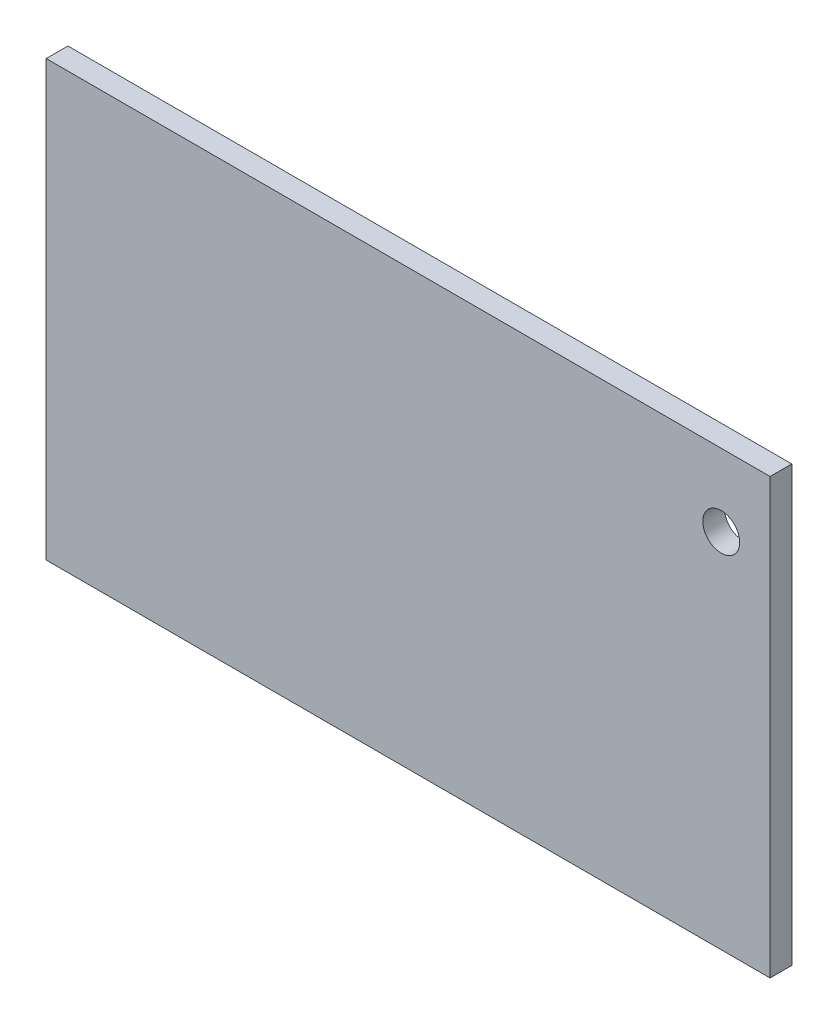
SolidWorks part; units mm, degrees
material "1023 碳钢板 (SS)"
ref_plane "Front Plane" through (0, 0, 0) normal (0, 0, 1) x (1, 0, 0)
ref_plane "Top Plane" through (0, 0, 0) normal (0, 1, 0) x (1, 0, 0)
ref_plane "Right Plane" through (0, 0, 0) normal (1, 0, 0) x (0, 0, -1)
sketch "Sketch1" plane through (0, 0, 0) normal (0, 0, 1) x (1, 0, 0)
  line L1 (100, 60) -> (-100, 60)
  line L2 (100, 60) -> (100, -60)
  line L3 (100, -60) -> (-100, -60)
  line L4 (-100, 60) -> (-100, -60)
  line L5 (100, 60) -> (-100, -60) construction
  line L6 (100, -60) -> (-100, 60) construction
  point P0 (0, 0)
  dimension "D1" = 200
  dimension "D2" = 120
extrude "Boss-Extrude1" add sketch "Sketch1" along normal blind 6
sketch "Sketch2" plane through (0, 0, 6) normal (0, 0, 1) x (1, 0, 0)
  line L0 (100, 60) -> (-100, 60) construction
  line L1 (100, -60) -> (100, 60) construction
  circle A0 centre (86.5, 40) radius 4.5
  dimension "D1" = 20
  dimension "D2" = 13.5
  dimension "D3" = 9
hole_wizard "M12 Tapped Hole1" positions "Sketch3" profile "Sketch4" tap size "M12" standard "ISO"
sketch "Sketch3" plane through (0, 0, 6) normal (0, 0, 1) x (1, 0, 0)
  point P0 (86.5, 40)
sketch "Sketch4" plane through (86.5, 40, 6) normal (1, 0, 0) x (0, -1, 0)
  line L0 (0, 0) -> (0, 32.3144)
  line L1 (0, 32.3144) -> (5.1, 29.25)
  line L2 (5.1, 29.25) -> (5.1, 0)
  line L5 (5.1, 0) -> (0, 0)
  line L10 (0, 32.3144) -> (-5.1, 29.25) construction
  line L11 (0, -6.35) -> (0, 107.95) construction
  dimension "螺纹孔钻头直径" = 10.2
  dimension "螺纹孔钻头深度" = 29.25
  dimension "导头角度" = 118
cosmetic thread "Hole Thread Line 1"
